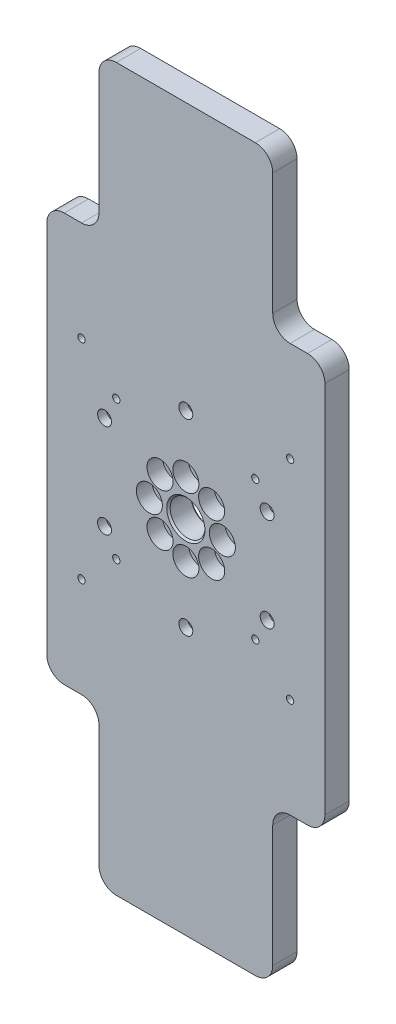
SolidWorks part; units mm, degrees
material "AL6061"
ref_plane "前视基准面" through (0, 0, 0) normal (0, 0, 1) x (1, 0, 0)
ref_plane "上视基准面" through (0, 0, 0) normal (0, 1, 0) x (1, 0, 0)
ref_plane "右视基准面" through (0, 0, 0) normal (1, 0, 0) x (0, 0, -1)
sketch "草图1" plane through (0, 0, 0) normal (0, 0, 1) x (1, 0, 0)
  line L0 (-148.0847, 0) -> (142.9639, 0) construction
  line L1 (0, 103.7016) -> (0, -118.6272) construction
  line L3 (-70, 117.5) -> (70, 117.5)
  line L4 (-80, 107.5) -> (-80, -107.5)
  line L5 (-70, -117.5) -> (70, -117.5)
  line L6 (80, 107.5) -> (80, -107.5)
  arc A0 (70, 117.5) -> (80, 107.5) centre (70, 107.5) cw
  arc A1 (-80, -107.5) -> (-70, -117.5) centre (-70, -107.5) ccw
  arc A2 (70, -117.5) -> (80, -107.5) centre (70, -107.5) ccw
  arc A3 (-70, 117.5) -> (-80, 107.5) centre (-70, 107.5) ccw
  circle A4 centre (0, 0) radius 10
  dimension "D3" = 10
  dimension "D4" = 20
  dimension "D1" = 160
  dimension "D2" = 235
extrude "凸台-拉伸1" add sketch "草图1" along normal mid plane 14
hole_wizard "打孔尺寸(%根据)内六角圆柱头螺钉的类型3" positions "草图2" profile "草图3" counterbore size "M8" standard "GB" end condition through all
sketch "草图2" plane through (0, 0, 7) normal (0, 0, 1) x (1, 0, 0)
  line L0 (0, 146.7369) -> (0, -120.7416) construction
  line L1 (0, 0) -> (0, 30.7954) construction
  circle A0 centre (0, 0) radius 21 construction
  point P0 (0, 21)
  dimension "D1" = 42
  dimension "D2" = 0
sketch "草图3" plane through (0, 21, 7) normal (1, 0, 0) x (0, -1, 0)
  line L0 (0, 0) -> (0, 14)
  line L1 (0, 14) -> (4.5, 14)
  line L3 (4.5, 14) -> (4.5, 9)
  line L4 (4.5, 9) -> (7.5, 9)
  line L5 (7.5, 9) -> (7.5, 0)
  line L7 (7.5, 0) -> (0, 0)
  line L11 (0, -6.35) -> (0, 107.95) construction
  dimension "通孔孔直径" = 9
  dimension "通孔孔深度" = 14
  dimension "柱形沉头孔直径" = 15
  dimension "柱形沉头孔深度" = 9
pattern_circular "阵列(圆周)1" count 8 over 360 about axis through (0, 0, 0) along (0, 0, 1) of "打孔尺寸(%根据)内六角圆柱头螺钉的类型3"
chamfer "倒角1" distance 1 angle 45 2 edges at (10, 0, -7) (10, 0, 7)
hole_wizard "Ø6.0 (6) 直径孔1" positions "草图8" profile "草图9" hole size "Ø6.0" standard "GB" end condition through all
sketch "草图8" plane through (0, 0, 7) normal (0, 0, 1) x (1, 0, 0)
  line L0 (0, 79.3748) -> (0, -57.9971) construction
  circle A0 centre (0, 0) radius 54 construction
  point P0 (0, 54)
  dimension "D1" = 108
sketch "草图9" plane through (0, 54, 7) normal (1, 0, 0) x (0, -1, 0)
  line L0 (0, 0) -> (0, 14)
  line L1 (0, 14) -> (3, 14)
  line L2 (3, 14) -> (3, 0)
  line L5 (3, 0) -> (0, 0)
  line L11 (0, -6.35) -> (0, 107.95) construction
  dimension "通孔孔直径" = 6
  dimension "通孔孔深度" = 14
sketch "草图14" plane through (0, 0, 7) normal (0, 0, 1) x (1, 0, 0)
  circle A0 centre (0, 54) radius 4
  dimension "D1" = 8
extrude "切除-拉伸1" cut sketch "草图14" against normal blind 5
hole_wizard "M5 螺纹孔1" positions "草图12" profile "草图13" tap size "M5" standard "GB" end condition through all
sketch "草图12" plane through (0, 0, 7) normal (0, 0, 1) x (1, 0, 0)
  line L0 (0, 144.6561) -> (0, -157.0077) construction
  line L1 (-143.9435, 0) -> (156.2951, 0) construction
  point P40 (-40, 40)
  point P43 (40, 40)
  point P45 (40, -40)
  point P46 (-40, -40)
  point P56 (-60, -60)
  point P85 (60, -60)
  point P88 (60, 60)
  point P93 (-60, 60)
  dimension "D1" = 120
  dimension "D2" = 120
  dimension "D5" = 80
  dimension "D6" = 80
sketch "草图13" plane through (-60, 60, 7) normal (1, 0, 0) x (0, -1, 0)
  line L0 (0, 0) -> (0, 14)
  line L1 (0, 14) -> (2.1, 14)
  line L2 (2.1, 14) -> (2.1, 0)
  line L5 (2.1, 0) -> (0, 0)
  line L11 (0, -6.35) -> (0, 107.95) construction
  dimension "通孔螺纹孔钻头直径" = 4.2
  dimension "通孔螺纹孔钻头深度" = 14
cosmetic thread "孔螺蚊线3" parameters "D2"=5
cosmetic thread "孔螺蚊线7" parameters "D2"=5
cosmetic thread "孔螺蚊线10" parameters "D2"=5
cosmetic thread "孔螺蚊线17" parameters "D2"=5
cosmetic thread "孔螺蚊线19" parameters "D2"=5
cosmetic thread "孔螺蚊线20" parameters "D2"=5
cosmetic thread "孔螺蚊线21" parameters "D2"=5
cosmetic thread "孔螺蚊线22" parameters "D2"=5
pattern_circular "阵列(圆周)2" count 6 over 360 about axis through (0, 0, 0) along (0, 0, 1) of "Ø6.0 (6) 直径孔1", "切除-拉伸1"
sketch "草图15" plane through (0, 0, 7) normal (0, 0, 1) x (1, 0, 0)
  line L0 (70, 117.5) -> (-70, 117.5) construction
  line L1 (-50, 117.5) -> (50, 117.5)
  line L2 (-50, 117.5) -> (-50, 207.5)
  line L3 (-50, 207.5) -> (50, 207.5)
  line L4 (50, 117.5) -> (50, 207.5)
  line L5 (0, 207.5) -> (0, 0) construction
  dimension "D1" = 100
  dimension "D2" = 90
extrude "凸台-拉伸2" add sketch "草图15" against normal up to surface (14 mm away) up to face at (49.7654, 27, -7)
mirror "镜向1" about plane through (0, 0, 0) normal (0, 1, 0) of "凸台-拉伸2"
fillet "圆角1" radius 10 8 edges at (50, 117.5, 0) (-50, 117.5, 0) (50, 207.5, 0) (-50, 207.5, 0) (50, -117.5, 0) (-50, -117.5, 0) (50, -207.5, 0) (-50, -207.5, 0)
